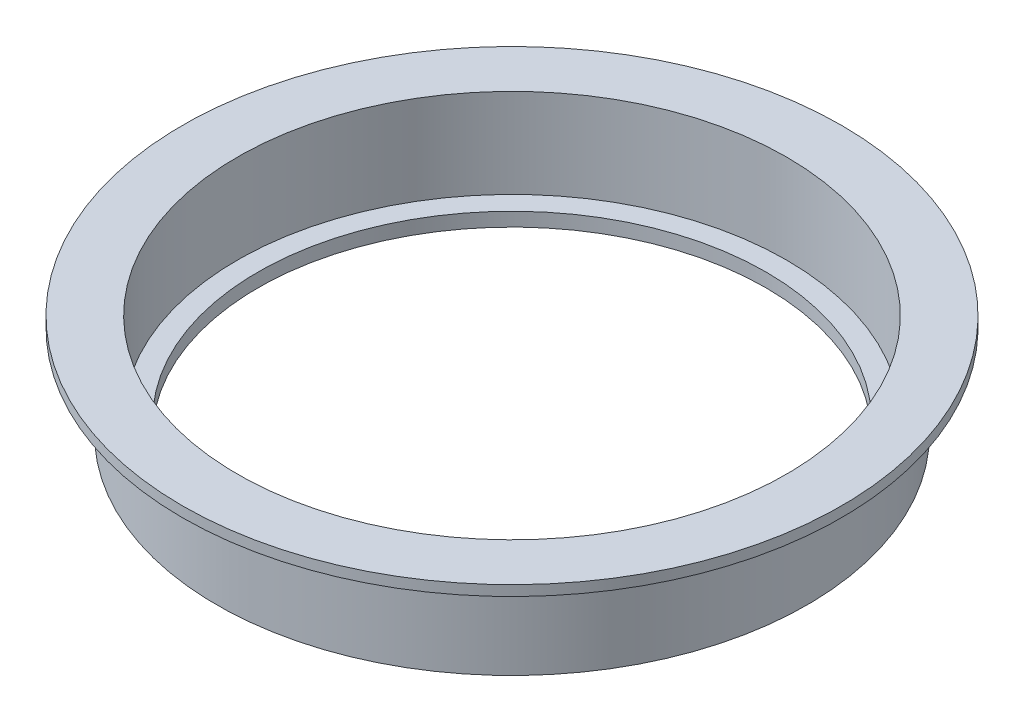
from build123d import *


with BuildPart() as part:
    # 草图1 → 旋转1 (revolve)
    with BuildSketch(Plane.XY, mode=Mode.PRIVATE) as revolve_1_sk:
        Polygon((-37, 0), (-37, 2), (-40, 2), (-40, 15), (-48, 15), (-48, 13.5), (-43, 13.5), (-43, 0), align=None)
    revolve(revolve_1_sk.sketch.rotate(Axis((0, 0, 0), (0, 1, 0)), 270), axis=Axis((0, 0, 0), (0, 1, 0)))


solid = part.part
